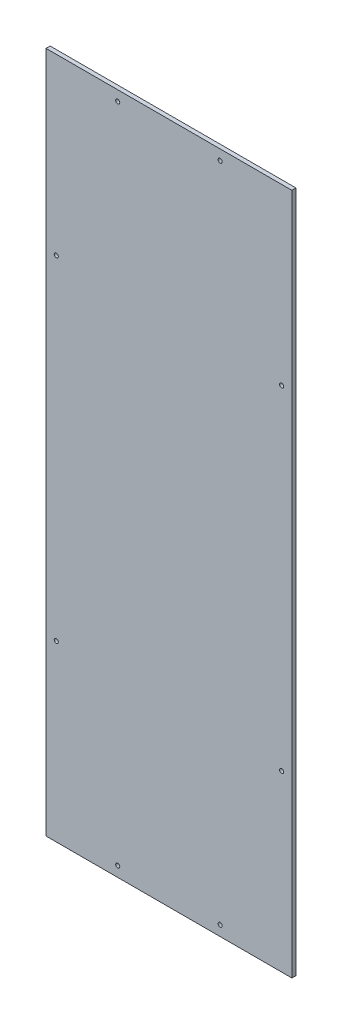
from build123d import *

# Parameters (mm, degrees)
SKETCH_1_W            = 240
SKETCH_1_H            = 666
EXTRUDE_1_DEPTH       = 2
HOLE_WIZARD_4_0_4_1_D = 4
HOLE_WIZARD_4_0_4_2_D = 4


with BuildPart() as part:
    # 草图1 → 凸台-拉伸1 (new, symmetric)
    with BuildSketch(Plane.XY):
        Rectangle(SKETCH_1_W, SKETCH_1_H)
    extrude(amount=EXTRUDE_1_DEPTH, both=True)

    # Ø4.0 (4) 直径孔1 (through all)
    with Locations(Plane(origin=(0, 0, -2), x_dir=(-1, 0, 0), z_dir=(0, 0, -1))):
        with Locations((-110, 163), (-110, -163)):
            hole_wizard_4_0_4_1 = Hole(HOLE_WIZARD_4_0_4_1_D / 2)

    # Ø4.0 (4) 直径孔2 (through all)
    with Locations(Plane(origin=(0, 0, -2), x_dir=(-1, 0, 0), z_dir=(0, 0, -1))):
        with Locations((-50, 323), (50, 323)):
            hole_wizard_4_0_4_2 = Hole(HOLE_WIZARD_4_0_4_2_D / 2)

    # 镜向1: Ø4.0 (4) 直径孔2 across plane
    add(hole_wizard_4_0_4_2.mirror(Plane.ZX), mode=Mode.SUBTRACT)

    # 镜向2: Ø4.0 (4) 直径孔1 across plane
    add(hole_wizard_4_0_4_1.mirror(Plane(origin=(0, 0, 0), x_dir=(0, 0, 1), z_dir=(1, 0, 0))), mode=Mode.SUBTRACT)


solid = part.part
